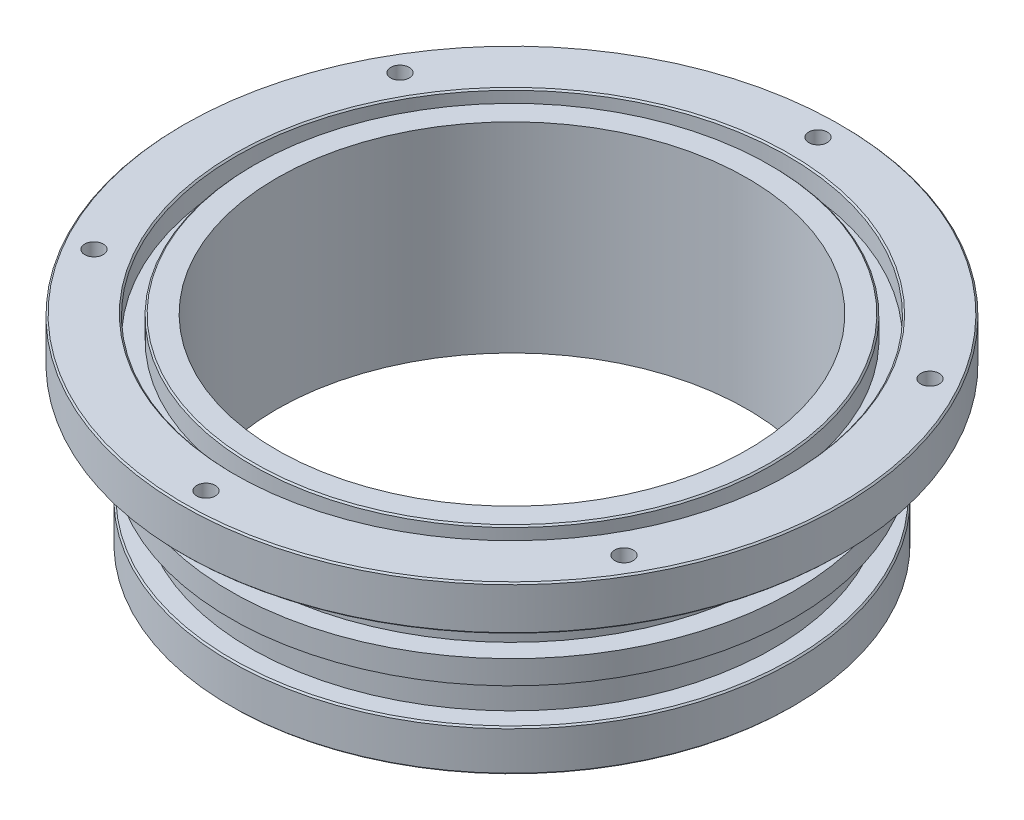
from build123d import *

# Parameters (mm, degrees)
CHAMFER_1_SIZE         = 0.2
HOLE_WIZARD_M3_1_D     = 2.5
HOLE_WIZARD_M3_1_DEPTH = 7.5
HOLE_WIZARD_M3_1_TIP   = 0.751075774
SKETCH_4_R             = 37.25
SKETCH_4_R_2           = 35
CUT_EXTRUDE_1_DEPTH    = 3
CHAMFER_2_SIZE         = 0.2


with BuildPart() as part:
    # 草图1 → 旋转1 (revolve)
    with BuildSketch(Plane.XY):
        Polygon((-31.75, 27), (-31.75, 0), (-37.973, 0), (-37.973, 5.587), (-35.2806, 5.587), (-35.2806, 10.413), (-37.973, 10.413), (-37.973, 13.587), (-35.2806, 13.587), (-35.2806, 18.413), (-37.973, 18.413), (-37.973, 21), (-44.45, 21), (-44.45, 27), align=None)
    revolve(axis=Axis((0, 27, 0), (0, -1, 0)))

    # 倒角1
    chamfer_1_edges = [part.edges().sort_by_distance(p)[0] for p in [
        (37.973, 5.587, 0),
        (37.973, 0, 0),
        (44.45, 27, 0),
        (44.45, 21, 0),
    ]]
    chamfer(chamfer_1_edges, length=CHAMFER_1_SIZE)

    # M3 螺纹孔1
    with Locations(Plane(origin=(0, 27, 0), x_dir=(1, 0, 0), z_dir=(0, 1, 0))):
        with Locations((-35.745198541, -20.6375), (-35.745198541, 20.6375), (0, 41.275), (35.745198541, 20.6375), (35.745198541, -20.6375), (0, -41.275)):
            Hole(HOLE_WIZARD_M3_1_D / 2, depth=HOLE_WIZARD_M3_1_DEPTH)
            with Locations((0, 0, -(HOLE_WIZARD_M3_1_DEPTH + HOLE_WIZARD_M3_1_TIP / 2))):  # 118° drill point
                Cone(0, HOLE_WIZARD_M3_1_D / 2, HOLE_WIZARD_M3_1_TIP, mode=Mode.SUBTRACT)

    # 草图4 → 切除-拉伸1 (cut)
    with BuildSketch(Plane(origin=(0, 27, 0), x_dir=(1, 0, 0), z_dir=(0, 1, 0))):
        with Locations(Location((0, 0, 0), (0, 0, 180))):
            Circle(SKETCH_4_R)
        with Locations(Location((0, 0, 0), (0, 0, 180))):
            Circle(SKETCH_4_R_2, mode=Mode.SUBTRACT)
    extrude(amount=-CUT_EXTRUDE_1_DEPTH, mode=Mode.SUBTRACT)

    # 倒角2
    chamfer_2_edges = [part.edges().sort_by_distance(p)[0] for p in [
        (37.25, 27, 0),
        (35, 27, 0),
    ]]
    chamfer(chamfer_2_edges, length=CHAMFER_2_SIZE)


solid = part.part
